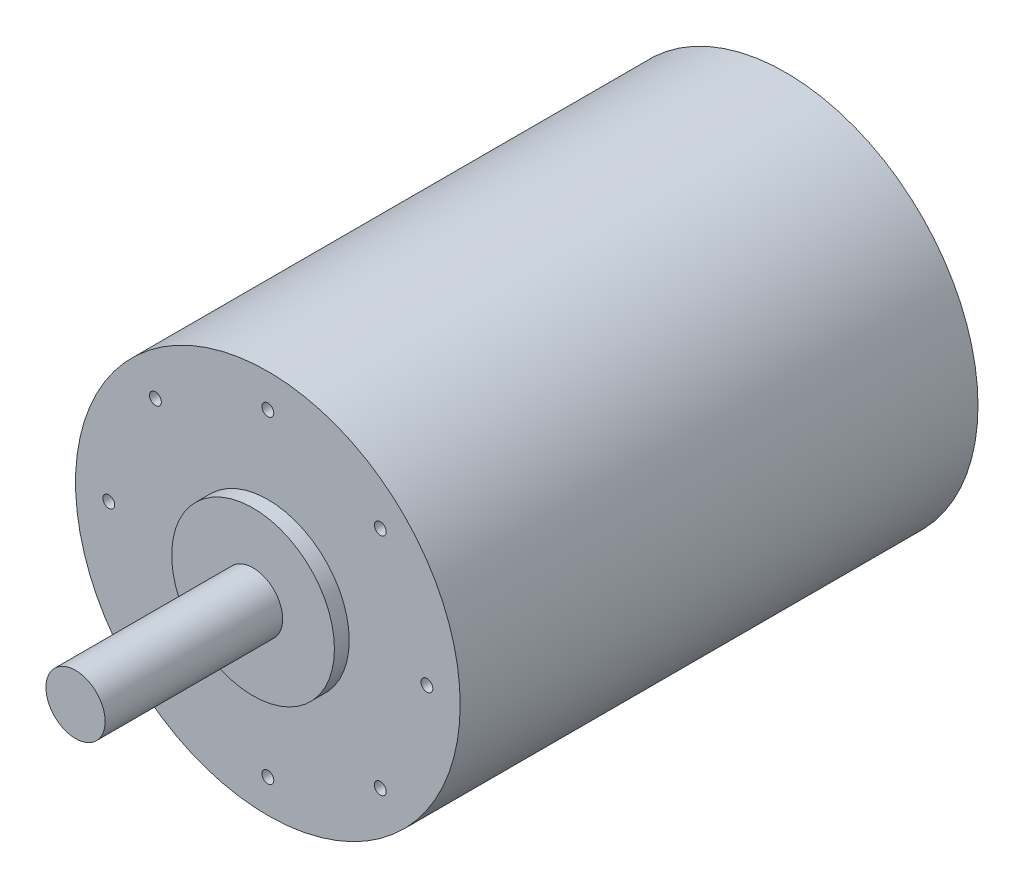
SolidWorks part; units mm, degrees
material "标准件"
ref_plane "前视基准面" through (0, 0, 0) normal (0, 0, 1) x (1, 0, 0)
ref_plane "上视基准面" through (0, 0, 0) normal (0, 1, 0) x (1, 0, 0)
ref_plane "右视基准面" through (0, 0, 0) normal (1, 0, 0) x (0, 0, -1)
sketch "草图1" plane through (0, 0, 0) normal (0, 0, 1) x (1, 0, 0)
  circle A0 centre (0, 0) radius 26
  dimension "D1" = 52
extrude "凸台-拉伸1" add sketch "草图1" along normal blind 70
sketch "草图2" plane through (0, 0, 70) normal (0, 0, 1) x (1, 0, 0)
  circle A0 centre (0, 0) radius 11
  dimension "D1" = 22
extrude "凸台-拉伸2" add sketch "草图2" along normal blind 2
sketch "草图3" plane through (0, 0, 72) normal (0, 0, 1) x (1, 0, 0)
  circle A0 centre (0, 0) radius 4
  dimension "D1" = 8
extrude "凸台-拉伸3" add sketch "草图3" along normal blind 24
hole_wizard "M2 螺纹孔1" positions "草图4" profile "草图5" tap size "M2" standard "ISO"
sketch "草图4" plane through (0, 0, 70) normal (0, 0, 1) x (1, 0, 0)
  line L0 (0, 21.5) -> (0, 0) construction
  line L1 (0, 0) -> (0, 21.5) construction
  point P0 (0, 21.5)
  point P8 (15.2028, 15.2028)
  point P9 (21.5, 0)
  point P10 (15.2028, -15.2028)
  point P11 (0, -21.5)
  point P12 (-15.2028, -15.2028)
  point P13 (-21.5, 0)
  point P14 (-15.2028, 15.2028)
  point P17 (0, -0.0498)
  dimension "D1" = 21.5
sketch "草图5" plane through (0, 21.5, 70) normal (1, 0, 0) x (0, -1, 0)
  line L0 (0, 0) -> (0, 5.6807)
  line L1 (0, 5.6807) -> (0.8, 5.2)
  line L2 (0.8, 5.2) -> (0.8, 0)
  line L5 (0.8, 0) -> (0, 0)
  line L10 (0, 5.6807) -> (-0.8, 5.2) construction
  line L11 (0, -6.35) -> (0, 107.95) construction
  dimension "螺纹孔钻头直径" = 1.6
  dimension "螺纹孔钻头深度" = 5.2
  dimension "导头角度" = 118
cosmetic thread "孔螺蚊线1" parameters "D1"=4, "D2"=2
cosmetic thread "孔螺蚊线2" parameters "D1"=4, "D2"=2
cosmetic thread "孔螺蚊线3" parameters "D1"=4, "D2"=2
cosmetic thread "孔螺蚊线4" parameters "D1"=4, "D2"=2
cosmetic thread "孔螺蚊线5" parameters "D1"=4, "D2"=2
cosmetic thread "孔螺蚊线6" parameters "D1"=4, "D2"=2
cosmetic thread "孔螺蚊线7" parameters "D1"=4, "D2"=2
cosmetic thread "孔螺蚊线8" parameters "D1"=4, "D2"=2
